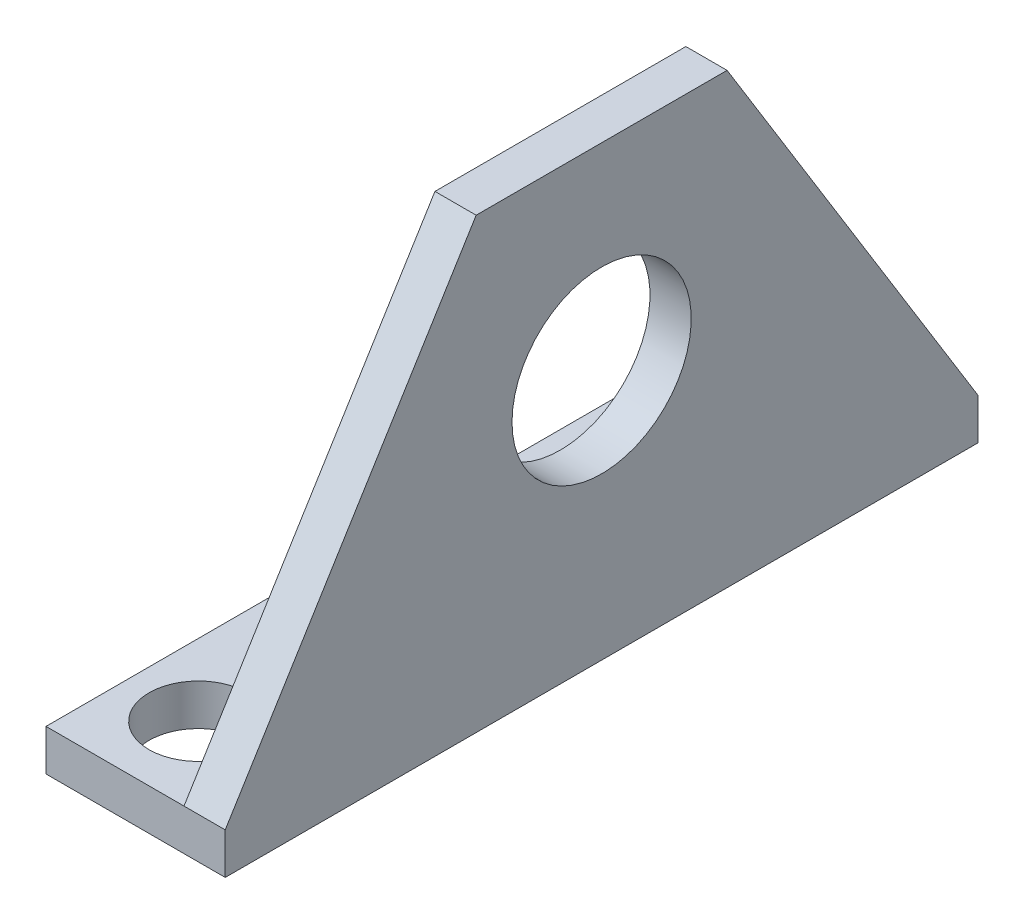
SolidWorks part; units mm, degrees
ref_plane "Front Plane" through (0, 0, 0) normal (0, 0, 1) x (1, 0, 0)
ref_plane "Top Plane" through (0, 0, 0) normal (0, 1, 0) x (1, 0, 0)
ref_plane "Right Plane" through (0, 0, 0) normal (1, 0, 0) x (0, 0, -1)
ref_plane "Plane1" through (-2.3, 0, 0) normal (-1, 0, 0) x (0, -1, 0)
sketch "Sketch1" plane through (-2.3, 0, 0) normal (-1, 0, 0) x (0, -1, 0)
  line L0 (11.7, 21) -> (-22.35, 0)
  line L1 (-22.35, 0) -> (11.7, -21)
  line L2 (11.7, -21) -> (14, -21)
  line L3 (14, -21) -> (14, 21)
  line L4 (14, 21) -> (11.7, 21)
extrude "Boss-Extrude1" add sketch "Sketch1" against normal blind 2.3
sketch "Sketch2" plane through (-2.3, 0, 0) normal (-1, 0, 0) x (0, 0, 1)
  line L0 (21, -11.7) -> (21, -14)
  line L1 (21, -14) -> (-21, -14)
  line L2 (-21, -14) -> (-21, -11.7)
  line L3 (-21, -11.7) -> (21, -11.7)
extrude "Boss-Extrude2" add sketch "Sketch2" along normal blind 7.7
hole_wizard "Ø10.0 (10) Diameter Hole1" positions "Sketch4" profile "Sketch3" hole size "Ø10.0" standard "ANSI Metric"
sketch "Sketch4" plane through (-2.3, 0, 0) normal (-1, 0, 0) x (0, 0, 1)
  point P0 (0, 0)
sketch "Sketch3" plane through (-2.3, 0, 0) normal (0, 1, 0) x (0, 0, 1)
  line L0 (0, 0) -> (0, 2.3)
  line L1 (0, 2.3) -> (5, 2.3)
  line L2 (5, 2.3) -> (5, 0)
  line L5 (5, 0) -> (0, 0)
  line L11 (0, -6.35) -> (0, 107.95) construction
  dimension "通孔孔直径" = 10
  dimension "通孔孔深度" = 2.3
hole_wizard "Ø5.5 (5.5) Diameter Hole1" positions "Sketch6" profile "Sketch5" hole size "Ø5.5" standard "ANSI Metric"
sketch "Sketch6" plane through (0, -11.7, 0) normal (0, 1, 0) x (1, 0, 0)
  point P0 (-6, -16.5)
  point P1 (-6, 16.5)
  dimension "D1" = 6
  dimension "D2" = 6
sketch "Sketch5" plane through (-6, -11.7, 16.5) normal (1, 0, 0) x (0, 0, 1)
  line L0 (0, 0) -> (0, 2.3)
  line L1 (0, 2.3) -> (2.75, 2.3)
  line L2 (2.75, 2.3) -> (2.75, 0)
  line L5 (2.75, 0) -> (0, 0)
  line L11 (0, -6.35) -> (0, 107.95) construction
  dimension "通孔孔直径" = 5.5
  dimension "通孔孔深度" = 2.3
chamfer "Chamfer1" distance 13.335 angle 58.336 1 edges at (-1.15, 22.35, 0)
